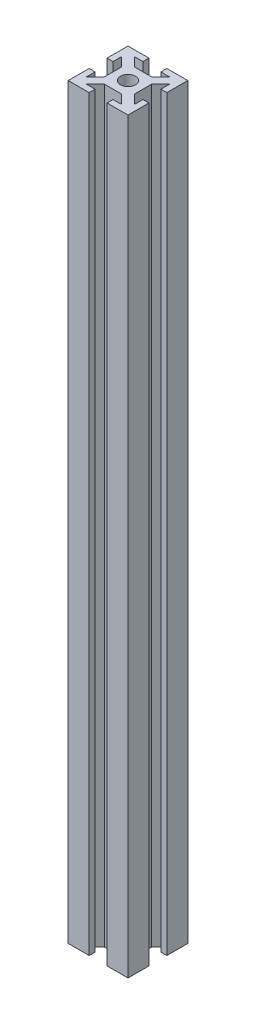
SolidWorks part; units mm, degrees
ref_plane "Front Plane" through (0, 0, 0) normal (0, 0, 1) x (1, 0, 0)
ref_plane "Top Plane" through (0, 0, 0) normal (0, 1, 0) x (1, 0, 0)
ref_plane "Right Plane" through (0, 0, 0) normal (1, 0, 0) x (0, 0, -1)
other "Configuration Table"
sketch "Sketch1" plane through (0, 0, 0) normal (0, 1, 0) x (1, 0, 0)
  line L0 (-6, 20) -> (-6, 16)
  line L5 (-20, 20) -> (-6, 20)
  line L6 (-20, 20) -> (-20, 6)
  line L7 (-20, -20) -> (-6, -20)
  line L8 (20, 20) -> (20, 6)
  line L9 (-20, 20) -> (20, -20) construction
  line L10 (-20, -20) -> (20, 20) construction
  line L11 (-6, 16) -> (-11.7574, 16)
  line L12 (-11.7574, 16) -> (-5.7574, 10)
  line L13 (5.7574, 10) -> (11.7574, 16)
  line L14 (11.7574, 16) -> (6, 16)
  line L15 (6, 16) -> (6, 20)
  line L16 (20, 6) -> (16, 6)
  line L17 (16, 6) -> (16, 11.7574)
  line L18 (16, 11.7574) -> (10, 5.7574)
  line L19 (10, -5.7574) -> (16, -11.7574)
  line L20 (16, -11.7574) -> (16, -6)
  line L21 (16, -6) -> (20, -6)
  line L22 (6, -20) -> (6, -16)
  line L23 (6, -16) -> (11.7574, -16)
  line L24 (11.7574, -16) -> (5.7574, -10)
  line L25 (-5.7574, -10) -> (-11.7574, -16)
  line L26 (-11.7574, -16) -> (-6, -16)
  line L27 (-6, -16) -> (-6, -20)
  line L28 (-20, -6) -> (-16, -6)
  line L29 (-16, -6) -> (-16, -11.7574)
  line L30 (-16, -11.7574) -> (-10, -5.7574)
  line L31 (-10, 5.7574) -> (-16, 11.7574)
  line L32 (-16, 11.7574) -> (-16, 6)
  line L33 (-16, 6) -> (-20, 6)
  line L34 (6, 20) -> (20, 20)
  line L35 (-20, -6) -> (-20, -20)
  line L36 (20, -6) -> (20, -20)
  line L37 (6, -20) -> (20, -20)
  line L39 (-5.7574, -10) -> (5.7574, -10)
  line L40 (-10, -5.7574) -> (-10, 5.7574)
  line L41 (-5.7574, 10) -> (5.7574, 10)
  line L42 (10, -5.7574) -> (10, 5.7574)
  line L43 (-10, -10) -> (10, 10) construction
  line L44 (-10, 10) -> (10, -10) construction
  circle A0 centre (0, 0) radius 5
  point P0 (0, 0)
  point P5 (0, 0)
  point P37 (0, 0)
  dimension "D10" = 10
  dimension "D1" = 40
  dimension "D2" = 4
  dimension "D3" = 4
  dimension "D4" = 14
  dimension "D5" = 14
  dimension "D6" = 3
  dimension "D7" = 3
  dimension "D8" = 4
  dimension "D9" = 20
extrude "Boss-Extrude1" add sketch "Sketch1" along normal blind 500
